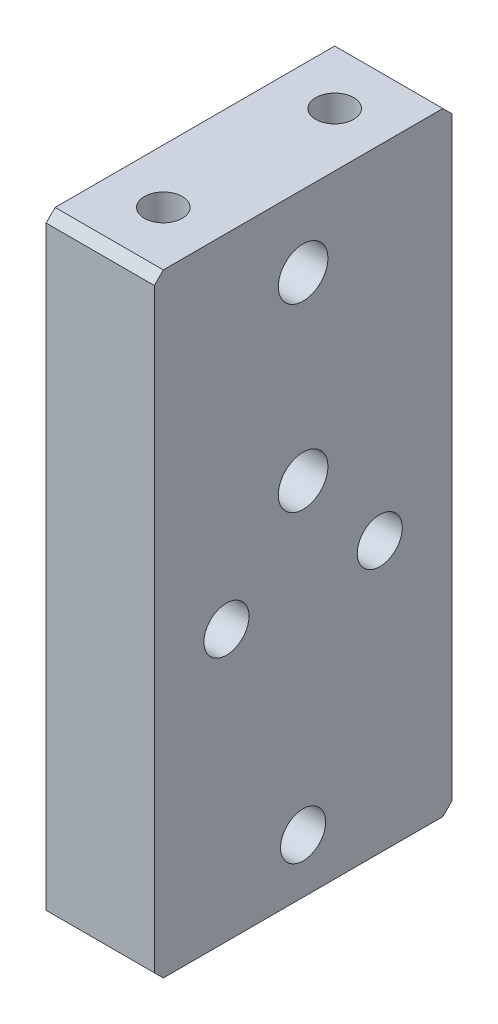
SolidWorks part; units mm, degrees
material "6061-T6 (SS)"
ref_plane "前视基准面" through (0, 0, 0) normal (0, 0, 1) x (1, 0, 0)
ref_plane "上视基准面" through (0, 0, 0) normal (0, 1, 0) x (1, 0, 0)
ref_plane "右视基准面" through (0, 0, 0) normal (1, 0, 0) x (0, 0, -1)
sketch "草图1" plane through (0, 0, 0) normal (0, 0, 1) x (1, 0, 0)
  line L1 (-76.4822, -79.6078) -> (-64.4822, -79.6078)
  line L2 (-76.4822, -79.6078) -> (-76.4822, -11.6078)
  line L3 (-76.4822, -11.6078) -> (-64.4822, -11.6078)
  line L4 (-64.4822, -79.6078) -> (-64.4822, -11.6078)
  dimension "D1" = 12
  dimension "D2" = 68
extrude "凸台-拉伸1" add sketch "草图1" against normal blind 33
hole_wizard "M6 螺纹孔1" positions "草图3" profile "草图4" tap size "M6" standard "Iso"
sketch "草图3" plane through (-76.4822, 0, 0) normal (-1, 0, 0) x (0, 0, 1)
  point P0 (-16.5, -73.6078)
  point P3 (-8, -49.6078)
  point P6 (-25, -49.6078)
sketch "草图4" plane through (-76.4822, -73.6078, -16.5) normal (0, 1, 0) x (0, 0, 1)
  line L0 (0, 0) -> (0, 16.5022)
  line L1 (0, 16.5022) -> (2.5, 15)
  line L2 (2.5, 15) -> (2.5, 0)
  line L5 (2.5, 0) -> (0, 0)
  line L10 (0, 16.5022) -> (-2.5, 15) construction
  line L11 (0, -6.35) -> (0, 107.95) construction
  dimension "螺纹孔钻头直径" = 5
  dimension "螺纹孔钻头深度" = 15
  dimension "导头角度" = 118
cosmetic thread "孔螺蚊线1"
cosmetic thread "孔螺蚊线2"
cosmetic thread "孔螺蚊线3"
hole_wizard "M5 螺纹孔1" positions "草图6" profile "草图5" tap size "M5" standard "Iso"
sketch "草图6" plane through (0, -11.6078, 0) normal (0, 1, 0) x (1, 0, 0)
  line L1 (-64.4822, 33) -> (-76.4822, 33) construction
  line L2 (-64.4822, 33) -> (-64.4822, 0) construction
  point P0 (-70.4822, 26)
  point P2 (-70.4822, 7)
  dimension "D1" = 19
  dimension "D2" = 7
  dimension "D3" = 6
sketch "草图5" plane through (-70.4822, -11.6078, -26) normal (1, 0, 0) x (0, 0, 1)
  line L0 (0, 0) -> (0, 12.2618)
  line L1 (0, 12.2618) -> (2.1, 11)
  line L2 (2.1, 11) -> (2.1, 0)
  line L5 (2.1, 0) -> (0, 0)
  line L10 (0, 12.2618) -> (-2.1, 11) construction
  line L11 (0, -6.35) -> (0, 107.95) construction
  dimension "螺纹孔钻头直径" = 4.2
  dimension "螺纹孔钻头深度" = 11
  dimension "导头角度" = 118
cosmetic thread "孔螺蚊线4"
cosmetic thread "孔螺蚊线5"
hole_wizard "打孔尺寸根据六角头螺栓 C 级的类型0" positions "草图8" profile "草图7" counterbore size "M5" standard "Gb" end condition through all
sketch "草图8" plane through (-76.4822, 0, 0) normal (-1, 0, 0) x (0, 0, 1)
  line L0 (0, -11.6078) -> (0, -79.6078) construction
  point P0 (-16.5, -19.6043)
  point P4 (-16.5, -39.6078)
  dimension "D1" = 16.5
sketch "草图7" plane through (-76.4822, -19.6043, -16.5) normal (0, 1, 0) x (0, 0, 1)
  line L0 (0, 0) -> (0, 12)
  line L1 (0, 12) -> (2.75, 12)
  line L3 (2.75, 12) -> (2.75, 5.5)
  line L4 (2.75, 5.5) -> (5, 5.5)
  line L5 (5, 5.5) -> (5, 0)
  line L7 (5, 0) -> (0, 0)
  line L11 (0, -6.35) -> (0, 107.95) construction
  dimension "通孔孔直径" = 5.5
  dimension "通孔孔深度" = 12
  dimension "柱形沉头孔直径" = 10
  dimension "柱形沉头孔深度" = 5.5
chamfer "倒角1" distance 1 angle 45 4 edges at (-70.4822, -11.6078, 0) (-70.4822, -11.6078, -33) (-70.4822, -79.6078, -33) (-70.4822, -79.6078, 0)
